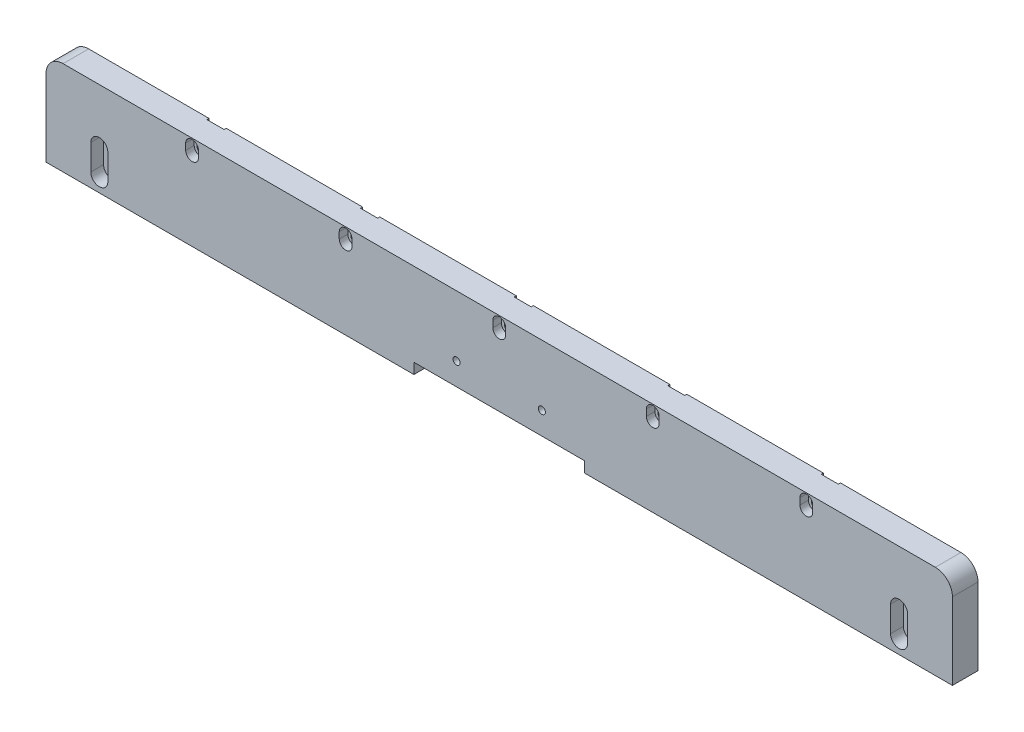
from build123d import *

# Parameters (mm, degrees)
SKETCH_1_W             = 425
SKETCH_1_H             = 44
EXTRUDE_1_DEPTH        = 12
FILLET_1_R             = 8
CUT_EXTRUDE_1_DEPTH    = 6
CUT_EXTRUDE_2_DEPTH    = 214.720027138
SKETCH_8_W             = 80
SKETCH_8_H             = 35.518481864
CUT_EXTRUDE_3_DEPTH    = 214.972544968
SKETCH_10_W            = 8
SKETCH_10_H            = 8.5
CUT_EXTRUDE_4_DEPTH    = 1
CUT_EXTRUDE_5_DEPTH    = 4
CUT_EXTRUDE_6_DEPTH    = 214.785523364
PATTERN_LINEAR_1_COUNT = 5
PATTERN_LINEAR_1_PITCH = 72
HOLE_WIZARD_M4_1_D     = 3.3


with BuildPart() as part:
    # 草图1 → 凸台-拉伸1 (new body)
    with BuildSketch(Plane.XY):
        Rectangle(SKETCH_1_W, SKETCH_1_H)
    extrude(amount=EXTRUDE_1_DEPTH)

    # 圆角1
    fillet_1_edges = [part.edges().sort_by_distance(p)[0] for p in [
        (-212.5, 22, 6),
        (212.5, 22, 6),
    ]]
    fillet(fillet_1_edges, radius=FILLET_1_R)

    # 草图2 → 切除-拉伸1 (cut)
    with BuildSketch(Plane.XY.offset(12)):
        with BuildLine():
            Line((-183.5, -3.5), (-183.5, -15.5))
            ThreePointArc((-183.5, -15.5), (-187.5, -19.5), (-191.5, -15.5))
            Line((-191.5, -15.5), (-191.5, -3.5))
            ThreePointArc((-191.5, -3.5), (-187.5, 0.5), (-183.5, -3.5))
        make_face()
        with BuildLine():
            Line((183.5, -3.5), (183.5, -15.5))
            ThreePointArc((183.5, -15.5), (187.5, -19.5), (191.5, -15.5))
            Line((191.5, -15.5), (191.5, -3.5))
            ThreePointArc((191.5, -3.5), (187.5, 0.5), (183.5, -3.5))
        make_face()
    extrude(amount=-CUT_EXTRUDE_1_DEPTH, mode=Mode.SUBTRACT)

    # 草图3 → 切除-拉伸2 (cut, through all)
    with BuildSketch(Plane.XY.offset(6)):
        with BuildLine():
            Line((-185.5, -3.5), (-185.5, -15.5))
            ThreePointArc((-185.5, -15.5), (-187.5, -17.5), (-189.5, -15.5))
            Line((-189.5, -15.5), (-189.5, -3.5))
            ThreePointArc((-189.5, -3.5), (-187.5, -1.5), (-185.5, -3.5))
        make_face()
        with BuildLine():
            Line((189.5, -3.5), (189.5, -15.5))
            ThreePointArc((189.5, -15.5), (187.5, -17.5), (185.5, -15.5))
            Line((185.5, -15.5), (185.5, -3.5))
            ThreePointArc((185.5, -3.5), (187.5, -1.5), (189.5, -3.5))
        make_face()
    extrude(amount=-CUT_EXTRUDE_2_DEPTH, mode=Mode.SUBTRACT)

    # 草图8 → 切除-拉伸3 (cut, through all)
    with BuildSketch(Plane.XY.offset(12)):
        with Locations((0, -34.759240932)):
            Rectangle(SKETCH_8_W, SKETCH_8_H)
    extrude(amount=-CUT_EXTRUDE_3_DEPTH, mode=Mode.SUBTRACT)

    # 草图10 → 切除-拉伸4 (cut)
    with BuildSketch(Plane(origin=(0, 0, 0), x_dir=(-1, 0, 0), z_dir=(0, 0, -1))):
        with Locations((-144, 17.75)):
            Rectangle(SKETCH_10_W, SKETCH_10_H)
        with Locations((-72, 17.75)):
            Rectangle(SKETCH_10_W, SKETCH_10_H)
        with Locations((0, 17.75)):
            Rectangle(SKETCH_10_W, SKETCH_10_H)
        with Locations((72, 17.75)):
            Rectangle(SKETCH_10_W, SKETCH_10_H)
        with Locations((144, 17.75)):
            Rectangle(SKETCH_10_W, SKETCH_10_H)
    extrude(amount=-CUT_EXTRUDE_4_DEPTH, mode=Mode.SUBTRACT)

    # 草图11 → 切除-拉伸5 (cut)
    with BuildSketch(Plane.XY.offset(12)):
        with BuildLine():
            Line((-141, 18.5), (-141, 15.5))
            ThreePointArc((-141, 15.5), (-144, 12.5), (-147, 15.5))
            Line((-147, 15.5), (-147, 18.5))
            ThreePointArc((-147, 18.5), (-144, 21.5), (-141, 18.5))
        make_face()
    cut_extrude_5 = extrude(amount=-CUT_EXTRUDE_5_DEPTH, mode=Mode.SUBTRACT)

    # 草图12 → 切除-拉伸6 (cut, through all)
    with BuildSketch(Plane.XY.offset(8)):
        with BuildLine():
            Line((-142.4, 18.5), (-142.4, 15.5))
            ThreePointArc((-142.4, 15.5), (-144, 13.9), (-145.6, 15.5))
            Line((-145.6, 15.5), (-145.6, 18.5))
            ThreePointArc((-145.6, 18.5), (-144, 20.1), (-142.4, 18.5))
        make_face()
    cut_extrude_6 = extrude(amount=-CUT_EXTRUDE_6_DEPTH, mode=Mode.SUBTRACT)

    # 阵列(线性)1: 切除-拉伸5, 切除-拉伸6 ×5
    with Locations(*[(i * PATTERN_LINEAR_1_PITCH, 0, 0) for i in range(1, PATTERN_LINEAR_1_COUNT)]):
        add(cut_extrude_5, mode=Mode.SUBTRACT)
        add(cut_extrude_6, mode=Mode.SUBTRACT)

    # M4 螺纹孔1 (through all)
    with Locations(Plane.XY.offset(12)):
        with Locations((-20, -6.5), (20, -6.5)):
            Hole(HOLE_WIZARD_M4_1_D / 2)


solid = part.part
